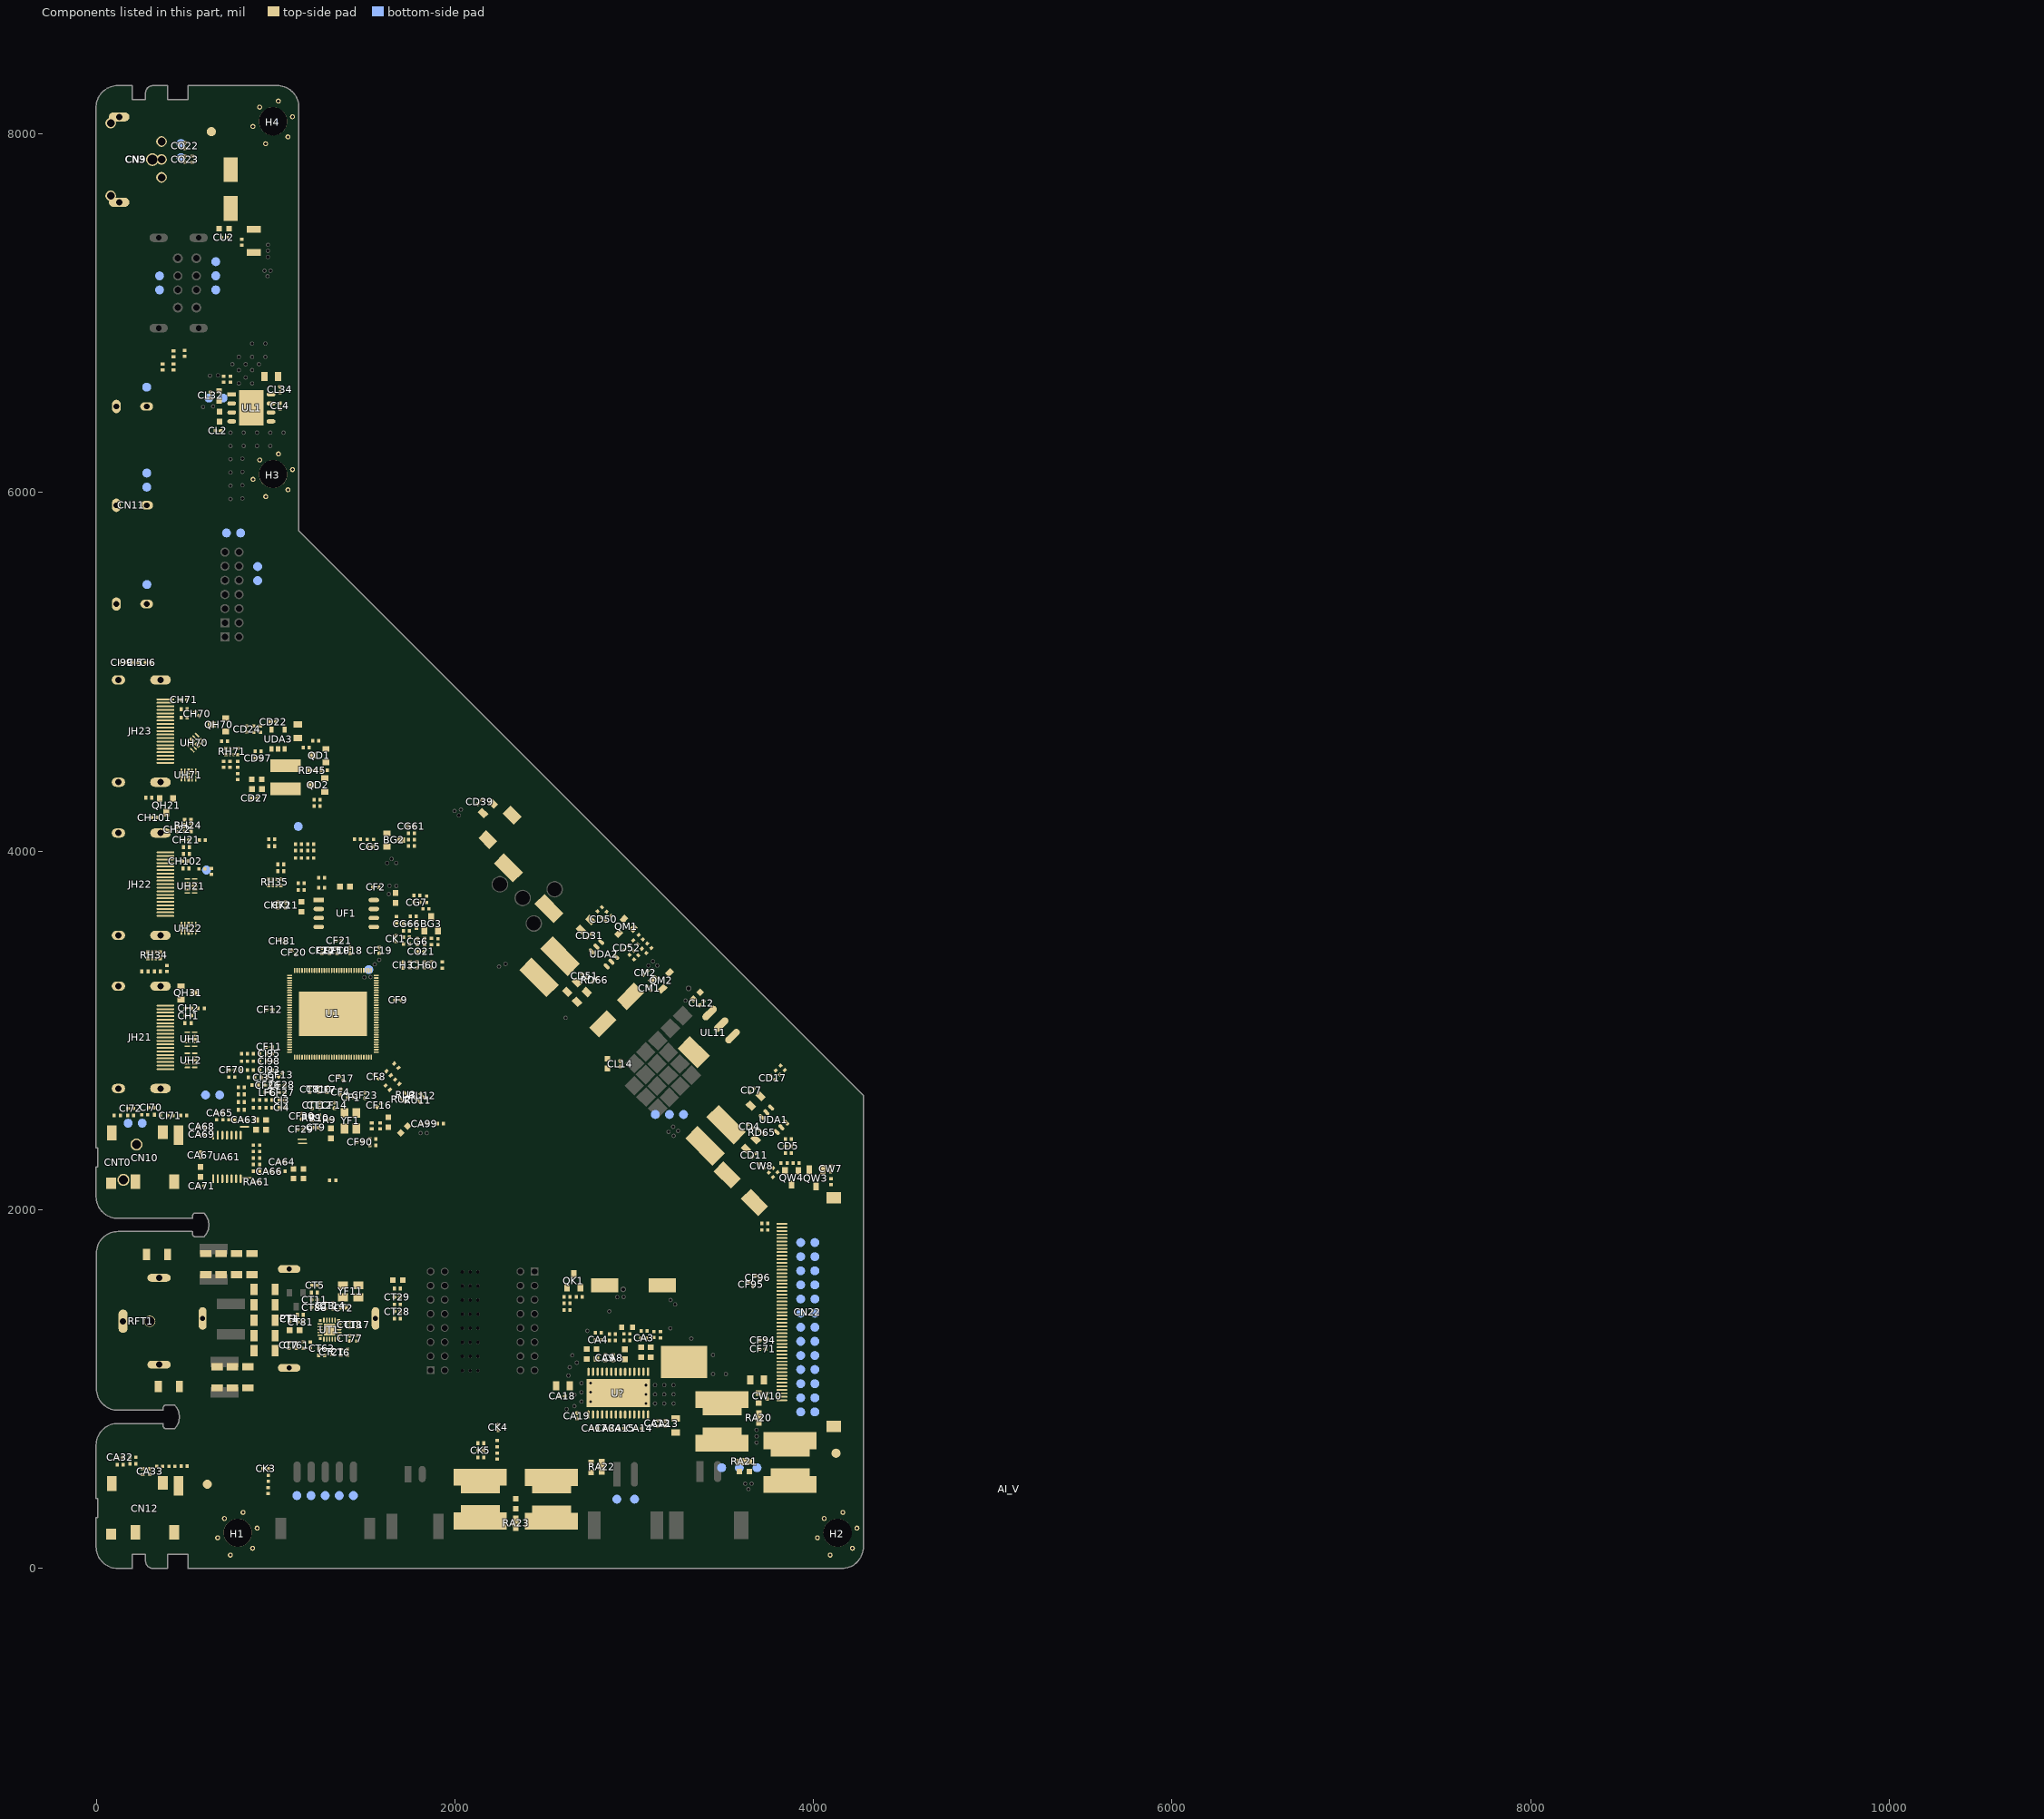
[diagram p0: the components of this part, seen from the top]
# Altium PCB MISC105950.PcbDoc (part 3 of 15)
Units mil, origin at the board's own origin, x right, y up, seen from the top; angles counter-clockwise.
Board outline 4280.62 x 8272.76 mil, 2 copper layers (TopLayer, BottomLayer), stack 61.855 mil thick; 541 components, 268 nets, 2324 pads, 1157 vias.

## Components (designator, comment, footprint, x,y, rotation, side; value= is the part's Value field where it differs from the comment) (continued)
LT4 "Ferrite bead,BEAD,1000ohm,0402,300mA,SMD,TRAY,CBM100505U102T,FH" L0402 1192.5,1243.5 r90 top
LT80 "NC/Multilayer inductor, HF Inductor, 270nH, ±5%, 0603, SMD, HCI1608F-R27J-M, Tai-tech" L0603 1105.5,1327 r0 top
M1 "MARK" MARK 617.5,467 r0 top
M2 "MARK" MARK 4125.5,640.5 r0 top
M3 "MARK" MARK 640,8013.5 r0 top
Manufacture_Info "Manufacture_Info" Manufacture_Info 2007.5,2940 r270 top
O0N "TEST" TP 4007.24,1815.64 r180 bottom
O0P "TEST" TP 3928.5,1815.64 r180 bottom
O1N "TEST" TP 4007.24,1736.9 r180 bottom
O1P "TEST" TP 3928.5,1736.9 r90 bottom
O2N "TEST" TP 4007.24,1658.16 r180 bottom
O2P "TEST" TP 3928.5,1658.16 r180 bottom
O3N "TEST" TP 4007.24,1500.68 r90 bottom
O3P "TEST" TP 3928.5,1500.68 r180 bottom
O4N "TEST" TP 4007.24,1421.94 r180 bottom
O4P "TEST" TP 3928.5,1421.94 r90 bottom
OCKN "TEST" TP 4007.24,1579.42 r90 bottom
OCKP "TEST" TP 3928.5,1579.42 r180 bottom
PT1 "NC/Shield cover, with seal, tinplate, T=0.3mm, natural color, 24.5×14×6mm, JLT" SHIELD(24.5*14*6)-TEMP-NG 1074,1392 r90 top locked
PWON "TEST" TP 898.43,5587.38 r90 bottom
QD1 "General-purpose transistor, Dynatron, PNP, 0.2A, 40V, 30-300, SOT-23, LMBT3906LT1G, LRC" SOT-23 1239.8,4532 r270 top
QD2 "General-purpose transistor, Dynatron, NPN, 0.2A, 40V, 30-300, SOT-23, LMBT3904LT1G, LRC" SOT-23 1233,4368.5 r270 top
QH21 "General-purpose transistor, Dynatron, NPN, 0.2A, 40V, 30-300, SOT-23, LMBT3904LT1G, LRC" SOT-23 389,4252.5 r0 top
QH31 "General-purpose transistor, Dynatron, NPN, 0.2A, 40V, 30-300, SOT-23, LMBT3904LT1G, LRC" SOT-23 511,3208.5 r90 top
QH70 "General-purpose transistor, Dynatron, NPN, 0.2A, 40V, 30-300, SOT-23, LMBT3904LT1G, LRC" SOT-23 680,4704.5 r270 top
QK1 "NC/MMBT3904(f≥350MHz)" SOT-23 2661.5,1602.5 r180 top
QM1 "General-purpose transistor, Dynatron, NPN, 0.2A, 40V, 30-300, SOT-23, LMBT3904LT1G, LRC" SOT-23 2940.5,3566 r315 top
QM2 "MOSFET, PMOS, -4.2A, -30V, 0.052ohm@ID=-4.2A@VGS=-10V, SOT-23-3, AO3401, BLUE ROCKET" SOT-23-1 3164,3290.5 r135 top
QW3 "MOSFET, PMOS, -4.3A, -30V, 0.048ohm@ID=-3A@VGS=-4.5V, SOT-23-3L, NCE3407AY, NCEPOWER" SOT-23-1 4013.84,2174.5 r0 top
QW4 "General-purpose transistor, Dynatron, NPN, 0.2A, 40V, 30-300, SOT-23, LMBT3904LT1G, LRC" SOT-23 3878,2176 r0 top
R9 "NC/0ohm-0402-PCB" R0402SC#2 1300,2500.5 r180 top
R10 "NC/0ohm-0402-PCB" R0402SC#1 1244,2511.77 r270 top
R99 "NC/0ohm-0402-PCB" R0402SC#1 1201.5,2511.77 r270 top
RA1 "4K7ohm-0402-±1%-1/16W" R0402 3145.5,1301 r270 top
RA2 "4K7ohm-0402-±1%-1/16W" R0402 3109,1301.5 r90 top
RA3 "1Kohm-0402-±1%-1/16W" R0402 3054,1322 r0 top
RA4 "NC/?" GND#1 1149.4,2368.34 r180 top
RA5 "NC/?" GND#1 1147.4,2392.34 r180 top
RA6 "Thick-film resistor, RES, 1/16W, 150ohm, ±1%, 0402, SMD" R0402 420.5,567.5 r180 top
RA7 "Thick-film resistor, RES, 1/10W, 200ohm, ±5%, 0603, SMD" R0603 2959.5,1342.5 r180 top
RA8 "100Kohm-0402-±1%-1/16W" R0402 2959.5,1306.5 r0 top
RA9 "NC/47Kohm-0402-±5%-1/16W" R0402 2959.5,1270 r0 top
RA10 "NC/10Kohm-0402-±1%-1/16W" R0402 2876.94,1269 r180 top
RA11 "NC/Thick-film resistor, RES, 1/16W, 13Kohm, ±1%, 0402, SMD" R0402 2876.94,1305.5 r180 top
RA14 "1Kohm-0402-±1%-1/16W" R0402 2799.02,1312.23 r180 top
RA15 "Thick-film resistor, RES, 1/16W, 150ohm, ±1%, 0402, SMD" R0402 203.5,580.5 r180 top
RA20 "NC/0ohm-0603-PCB" R0603SC 3694.5,837.5 r270 top
RA21 "NC/0ohm-0603-PCB" R0603SC 3612.5,594 r180 top
RA22 "NC/0ohm-0603-PCB" R0603SC 2818,565 r90 top
RA23 "NC/0ohm-0603-PCB" R0603SC 2339,250.22 r270 top
RA51 "47Kohm-0402-±1%-1/16W" R0402 957.5,432.5 r90 top
RA52 "10Kohm-0402-±1%-1/16W" R0402 1919,2478.5 r180 top
RA55 "1Kohm-0402-±1%-1/16W" R0402 203.5,618 r180 top
RA56 "1Kohm-0402-±1%-1/16W" R0402 352.5,567 r180 top
RA61 "NC/NC/0ohm-0402-PCB" R0402SC#1 892.5,2155 r180 top
RA62 "NC/47Kohm-0402-±5%-1/16W" R0402 755,2501 r180 top
RA63 "NC/47Kohm-0402-±5%-1/16W" R0402 1035,2213.5 r180 top
RA64 "NC/" GND#2 825.16,2461.54 r0 top
RA65 "NC/" GND#1 841,2176 r0 top
RA66 "NC/100Kohm-0402-±5%-1/16W" R0402 687.5,2501 r180 top
RA67 "NC/100Kohm-0402-±5%-1/16W" R0402 892.5,2213.5 r180 top
RA68 "NC/1Kohm-0402-±5%-1/16W" R0402 892.5,2323.75 r180 top
RA69 "NC/4K7ohm-0402-±5%-1/16W" R0402 892.5,2359.25 r180 top
RA70 "NC/12Kohm-0402-±5%-1/16W" R0402 1317.5,2162.5 r0 top
RA71 "NC/5K1ohm-0402-±5%-1/16W" R0402 892.5,2251.5 r0 top
RA72 "NC/12Kohm-0402-±5%-1/16W" R0402 892.5,2287.5 r180 top
RD1 "NC/10Kohm-0402-±5%-1/16W" R0402 3800.48,2764.52 r315 top
RD2 "100Kohm-0402-±1%-1/16W" R0402 900.27,4556.5 r0 top
RD28 "NC/4K7ohm-0402-±1%-1/16W" R0402 3827.15,2790.35 r135 top
RD31 "NC/Thick-film resistor, RES, 1/16W, 200Kohm, ±1%, 0402, SMD" R0402 3858.83,2314.54 r180 top
RD35 "NC/Thick-film resistor, RES, 1/16W, 10.5Kohm, ±1%, 0402, SMD" R0402 3859.27,2393 r0 top
RD42 "510ohm-0402-±1%-1/16W" R0402 1222,4615 r180 top
RD43 "4K7ohm-0402-±1%-1/16W" R0402 1170.27,4576.5 r0 top
RD44 "10Kohm-0402-±1%-1/16W" R0402 1271.3,4450 r180 top
RD45 "NC/0ohm-0402-PCB" R0402SC#1 1203.57,4450 r0 top
RD46 "10Kohm-0402-±1%-1/16W" R0402 1230.5,4251 r180 top
RD47 "NC/10Kohm-0402-±5%-1/16W" R0402 1230.5,4287 r0 top
RD52 "100Kohm-0402-±1%-1/16W" R0402 2807,3675 r45 top
RD53 "NC/Thick-film resistor, RES, 1/16W, 10Kohm, ±1%, 0402, SMD" R0402 2857.5,3649.5 r315 top
RD54 "Thick-film resistor, RES, 1/16W, 20Kohm, ±1%, 0402, SMD" R0402 3010,3406 r45 top
RD65 "NC/0ohm-0402-PCB" R0402SC#1 3711.5,2430.5 r315 top
RD66 "NC/0ohm-0402-PCB" R0402SC#1 2778,3279.5 r45 top
RD81 "12Kohm-0402-±1%-1/16W" R0402 877,4680 r270 top
RD88 "13Kohm-0402-±1%-1/16W" R0402 913,4680 r90 top
RD91 "Thick-film resistor, RES, 1/16W, 150Kohm, ±1%, 0402, SMD" R0402 2984.72,3432.6 r45 top
RF3 "NC/4K7ohm-0402-±5%-1/16W" R0402 1255,3795.5 r180 top
RF4 "NC/100ohm-0402-±5%-1/16W" R0402 3728,1922.27 r180 top
RF5 "NC/1Kohm-0402-±5%-1/16W" R0402 3728,1886 r0 top
RF12 "68ohm-0402-±5%-1/16W" R0402 884.5,2695 r180 top
RF13 "4K7ohm-0402-±1%-1/16W" R0402 1728.5,3518.5 r0 top
RF19 "68ohm-0402-±5%-1/16W" R0402 755,2738.5 r0 top
RF29 "4K7ohm-0402-±1%-1/16W" R0402 1766.5,3636.5 r180 top
RF43 "4K7ohm-0402-±1%-1/16W" R0402 1542.23,2393.5 r0 top
RF44 "4K7ohm-0402-±1%-1/16W" R0402 1542.23,2357.5 r0 top
RFT1 "RF connector, RF JACK, H, IEC, T14.5, CH6.3, with pipe, 23.8×15.1×11.9mm, SMD, 120-XX1, GD" T-12.8×10×9.3-IEC14.5-6.3 0.05,1376.72 r270 top locked
RG1 "10Kohm-0402-±1%-1/16W" R0402 1527.5,4064.5 r180 top
RG2 "NC/10Kohm-0402-±5%-1/16W" R0402 1784.5,3585 r270 top
RG3 "1Kohm-0402-±1%-1/16W" R0402 1729,3555.5 r180 top
RG6 "100ohm-0402-±1%-1/16W" R0402 1756.5,4063.75 r180 top
RG7 "NC/100ohm-0402-±5%-1/16W" R0402 1841,3730.5 r270 top
RG8 "NC/?" R0402 1756.5,4099.5 r0 top
RG9 "NC/NC/?" R0402 1786.5,3752 r0 top
RG29 "4K7ohm-0402-±1%-1/16W" R0402 1454.5,4065.5 r180 top
RG66 "1Kohm-0402-±1%-1/16W" R0402 1756.5,4028 r0 top
RG67 "NC/1Kohm-0402-±5%-1/16W" R0402 1838,3677.5 r180 top
RH1 "22Kohm-0402-±1%-1/16W" R0402 1929,3364 r90 top
RH2 "33Kohm-0402-±1%-1/16W" R0402 1868.5,3364.5 r90 top
RH23 "1Kohm-0402-±1%-1/16W" R0402 590.5,4061.5 r180 top
RH24 "Resistor array, RES ARRAY, 1/16W, 4×10Kohm, ±5%, 0402, SMD" RA0402 509.22,4142.34 r180 top
RH33 "1Kohm-0402-±1%-1/16W" R0402 583.5,3123 r0 top
RH34 "Resistor array, RES ARRAY, 1/16W, 4×10Kohm, ±5%, 0402, SMD" RA0402 320.54,3418.78 r270 top
RH35 "Resistor array, RES ARRAY, 1/16W, 4×33ohm, ±5%, 0402, SMD" RA0402 994,3826.5 r270 top
RH70 "1Kohm-0402-±1%-1/16W" R0402 714.5,4612 r180 top
RH71 "Resistor array, RES ARRAY, 1/16W, 4×10Kohm, ±5%, 0402, SMD" RA0402 754.34,4555.78 r90 top
RH72 "33ohm-0402-±1%-1/16W" R0402 708.5,4483 r270 top
RH73 "33ohm-0402-±1%-1/16W" R0402 744.5,4483 r270 top
RH74 "22Kohm-0402-±1%-1/16W" R0402 787.75,4483.26 r90 top
RH75 "33Kohm-0402-±1%-1/16W" R0402 787.75,4415.76 r270 top
RH81 "22Kohm-0402-±1%-1/16W" R0402 1786,3365.5 r90 top
RH82 "33Kohm-0402-±1%-1/16W" R0402 1749.5,3364.5 r90 top
RH83 "100ohm-0402-±1%-1/16W" R0402 587.5,3900 r180 top
RH101 "4K7ohm-0402-±1%-1/16W" R0402 1126.43,4002 r0 top
RH102 "Thick-film resistor, RES, 1/16W, 1.2Kohm, ±1%, 0402, SMD" R0402 1126.43,4037.75 r0 top
RH103 "1Kohm-0402-±1%-1/16W" R0402 1126.93,3961.25 r0 top
RH104 "4K7ohm-0402-±1%-1/16W" R0402 1194.43,3961.25 r0 top
RH105 "Thick-film resistor, RES, 1/16W, 220ohm, ±1%, 0402, SMD" R0402 1193.93,4037.75 r0 top
RH106 "NC/4K7ohm-0402-±5%-1/16W" R0402 1193.93,4002 r180 top
RI13 "10Kohm-0402-±1%-1/16W" R0402 892.5,2610 r180 top
RI14 "12Kohm-0402-±1%-1/16W" R0402 962.74,2610 r180 top
RI15 "10Kohm-0402-±1%-1/16W" R0402 892.5,2568 r180 top
RI16 "12Kohm-0402-±1%-1/16W" R0402 962.74,2568 r180 top
RI21 "75ohm-0402-±1%-1/16W" R0402 807,2682.5 r0 top
RI22 "33ohm-0402-±1%-1/16W" R0402 864.5,2736.5 r0 top
RI23 "75ohm-0402-±1%-1/16W" R0402 824.77,2869 r0 top
RI24 "33ohm-0402-±1%-1/16W" R0402 892,2869 r0 top
RI25 "75ohm-0402-±1%-1/16W" R0402 824.77,2778.5 r0 top
RI26 "33ohm-0402-±1%-1/16W" R0402 892,2778.5 r0 top
RI36 "75ohm-0402-±1%-1/16W" R0402 824.77,2827.5 r0 top
RI38 "33ohm-0402-±1%-1/16W" R0402 892,2827.5 r0 top
RI62 "Thick-film resistor, RES, 1/16W, 0ohm, ±1%, 0402, SMD" R0402 189,2524.5 r0 top
RI63 "Thick-film resistor, RES, 1/16W, 0ohm, ±1%, 0402, SMD" R0402 267.5,2528.5 r180 top
RK1 "22ohm-0402-±1%-1/16W" R0402 958,500 r90 top
RK2 "4K7ohm-0402-±1%-1/16W" R0402 2235.5,694 r270 top
RK6 "1Kohm-0402-±1%-1/16W" R0402 1673.5,3617 r270 top
RK10 "NC/1Kohm-0402-±5%-1/16W" R0402 2692.5,1512.5 r0 top
RK13 "NC/33Kohm-0402-±5%-1/16W" R0402 2624,1440 r0 top
RK14 "510ohm-0402-±1%-1/16W" R0402 2624.5,1512.5 r0 top
RK15 "NC/10Kohm-0402-±5%-1/16W" R0402 2624.5,1476.5 r0 top
RK23 "1Kohm-0402-±1%-1/16W" R0402 1255,3850 r0 top
RK25 "10Kohm-0402-±1%-1/16W" R0402 2235.5,624 r270 top
RL31 "120ohm-0402-±1%-1/16W" R0402 709.5,6632 r90 top
RL32 "200ohm-0402-±1%-1/16W" R0402 746.5,6632 r270 top
RM1 "10Kohm-0402-±1%-1/16W" R0402 3083.5,3471.5 r315 top
RM2 "10Kohm-0402-±1%-1/16W" R0402 3036.5,3519.5 r135 top
RM3 "4K7ohm-0402-±1%-1/16W" R0402 3006.5,3490.5 r315 top
RM4 "100Kohm-0402-±1%-1/16W" R0402 3054.5,3443 r315 top
RO21 "Thick-film resistor, RES, 1/16W, 150ohm, ±1%, 0402, SMD" R0402 1830,3495.5 r90 top
RO22 "NC/Thick-film resistor, RES, 1/16W, 75ohm, ±1%, 0402, SMD" R0402 1904.5,3495 r270 top
RO31 "Thick-film resistor, RES, 1/16W, 0ohm, ±1%, 0402, SMD" R0402 534,7859.38 r270 top
ROUT+ "DM0" TP 2902.57,384 r90 bottom
ROUT- "DM0" TP 3001,384 r90 bottom
RT1 "Thick-film resistor, RES, 1/16W, 51Kohm, ±1%, 0402, SMD" R0402 1255.5,1185.5 r180 top
RT2 "33ohm-0402-±1%-1/16W" R0402 1401,1204.5 r90 top
RT3 "33ohm-0402-±1%-1/16W" R0402 1452,1282 r90 top
RT4 "100ohm-0402-±1%-1/16W" R0402 1678.5,1391.5 r0 top
RT5 "100ohm-0402-±1%-1/16W" R0402 1677.5,1470.5 r0 top
RU1 "Thick-film resistor, RES, 1/16W, 0ohm, ±1%, 0402, SMD" R0402 809.38,7397.5 r270 top
RU2 "NC/0ohm-0402-PCB" R0402SC#1 1702.86,2614.64 r315 top
RU3 "NC/0ohm-0402-PCB" R0402SC#1 1728.38,2640.16 r315 top
RU11 "NC/0ohm-0402-PCB" R0402SC#1 1794.04,2608.96 r315 top
RU12 "NC/0ohm-0402-PCB" R0402SC#1 1819.33,2634.26 r315 top
RW10 "4K7ohm-0402-±1%-1/16W" R0402 3786.5,2219.5 r315 top
RW11 "NC/4K7ohm-0402-±5%-1/16W" R0402 4097.5,2156 r270 top
RW12 "47Kohm-0402-±1%-1/16W" R0402 3761.76,2193.47 r135 top
RW13 "4K7ohm-0402-±1%-1/16W" R0402 3835.27,2259.5 r0 top
RW14 "4K7ohm-0402-±1%-1/16W" R0402 3902.77,2259.5 r0 top
RXD "" TP 1125,4137.5 r270 bottom
S/N1 "Barcode" Barcode 2330.5,2498.5 r270 top
S/N2 "Barcode" Barcode 2465,2517 r90 bottom
SPDIF_OUT "TEST" TP 470.87,7947.38 r90 bottom
TXD "" TP 613,3894 r270 bottom
U1 "Customer-supplied TV main IC, IC Main Chip, SMD, TSUMV53RWU-Z1, COMPANY_A-ODM, MTK" QFN128/0.35-1 1318.5,3091.88 r0 top locked
U? "Audio amplifier, IC Audio, Class D, 2x10W@13V@8ohm, HTSSOP-28, SMD, CS3817EO, SEMICO" SSOP28/0.65-5 2910.2,975.41 r270 top
UA61 "NC/Audio amplifier, IC Headphone AMP, Class AB, 2×20mW@2.3V@32ohm, TSSOP-14, SMD, AD22653B-QH14NAR, ESMT" SSOP14/0.65-1 727.18,2293.06 r180 top locked
UDA1 "NC/DC-DC IC, IC DC-DC, Syn, 2A, 18V, 500kHz, SOT23-6, SMD, SM8102ABC, Silergy" SOT23-6-2 3778.5,2500.5 r45 top locked
UDA2 "DC-DC IC, IC DC-DC, Syn, 2A, 18V, 500kHz, SOT23-6, SMD, SM8102ABC, Silergy" SOT23-6-2 2830.5,3424.5 r45 top
UDA3 "DC-DC IC, IC DCDC, Syn, 1.2A, 6.0V, 1.5MHz, SOT23-5, SMD, TMI3408, TOLL" SOT-23-5 1012.5,4623.5 r0 top
UF1 "SPI flash IC, IC SPI FLASH, 4MB, 32Mb, SOIC8, SMD, W25Q32JVSSIQ, Winbond" SOIC8 1393.04,3651.5 r0 top locked
UH1 "NC/TVS diode, DIO ESD, 0.4pF, 19V, DFN2510-10L, SMD, ESD5304D-10/TR, Willsemi" RCL0524P 527,2950.38 r270 top
UH2 "NC/TVS diode, DIO ESD, 0.4pF, 19V, DFN2510-10L, SMD, ESD5304D-10/TR, Willsemi" RCL0524P 527,2832.38 r270 top
UH21 "NC/TVS diode, DIO ESD, 0.4pF, 19V, DFN2510-10L, SMD, ESD5304D-10/TR, Willsemi" RCL0524P 527,3804.71 r270 top
UH22 "NC/TVS diode, DIO ESD, 0.4pF, 19V, DFN2510-10L, SMD, ESD5304D-10/TR, Willsemi" RCL0524P 512.98,3569.5 r180 top
UH70 "NC/TVS diode, DIO ESD, 0.4pF, 19V, DFN2510-10L, SMD, ESD5304D-10/TR, Willsemi" RCL0524P 546.7,4605.01 r225 top
UH71 "NC/TVS diode, DIO ESD, 0.4pF, 19V, DFN2510-10L, SMD, ESD5304D-10/TR, Willsemi" RCL0524P 512.98,4423.83 r180 top
UL1 "LDO IC, IC LDO, 1A, 3.3V+ADJ, 12V, ESOP-8, SMD, LC1118CS8TRAD33, Leadchip" SOP8/1.27-3 863.5,6472 r0 top locked
UL11 "LDO IC, IC LDO, 1A, 1.8V, 15V, SOT-223, SMD, SCJT1117B-1.8V, CJKJ" SOT-223 3407.5,2955 r135 top
UT1 "Silicon tuner IC, IC Si Tuner, QFN-24, SMD, ATBM253, AltoBeam" QFN24/0.4-1 1299.5,1330 r90 top
VCC_CORE "TEST" TP 1518.5,3338.5 r315 bottom
VCC_PANEL1 "TEST" TP 3928.5,870.76 r90 bottom
XX.XXXX "PCB_NAME" PCB_NAME 1624.98,1044.62 r90 top
XXXXXX "PCB_TIME" PCB_TIME 8963.88,-1096.65 r90 top
XXXXXX. "PCB_TIME" PCB_TIME 1613.17,1044.62 r90 top
XXXXXXXX "PCB_NAME" PCB_NAME 8987.5,-1096.65 r90 top
XXXXXXXXXX "PCB_NAME" PCB_NAME 8952.07,-1096.65 r90 top
YF1 "Passive crystal oscillator, SPXO, 24MHz, ±10ppm, 12pF, SMD3225, SMD, SX32Y024000BC1T-Z, TKD" XTAL-S-3 1416.04,2495.51 r90 top
YF11 "Passive crystal oscillator, SPXO, 24MHz, ±10ppm, 12pF, SMD3225, SMD, SX32Y024000BC1T-Z, TKD" XTAL-S-3 1417,1543.5 r180 top locked
YPbPr_GND "TEST" TP 686.74,2639 r180 bottom
YPbPr_Pb "TEST" TP 254.5,2481.5 r180 bottom
YPbPr_Pr "TEST" TP 608,2639 r180 bottom
YPbPr_Y "TEST" TP 175.76,2481.5 r180 bottom
用U1上 "Glue, 0.1g, silicone, ZJ" "Heat-Shrinkable Tube" 8975.69,-1096.65 r90 top

## Footprints (in the part's own frame and the unit in brackets; to place one, negate y for a bottom-side part, rotate by r counter-clockwise, add the part's x,y. Pads: shape width x height; smd on the part's side, far side on the other; paste and mask are expansions set on the pad)
AI_GRIPPER_V [mm] "3D shape for vertical type AI equipment"
  round 1.5 on Mech5: 0(0,-2.5) 1(0,0) 2(0,2.5)
  body extent -29.13,-4.7 2.5,4.7, height 54.74
ASSE4.0C-3 [mm] "定位孔(顶底层上锡)(17.12.09更新过孔位置）18.11.22 更新paste形状为扇形。"
  round 4 hole 4 unplated mask+0: 0(0,0)
  round 0.7 hole 0.4: 1(-2.85,-0.725) 2(-1.893,2.011) 3(0.75,2.875) 4(2.75,0.65) 5(2.105,-2.203) 6(-1.05,-3.175)
  KeepOutLayer pour cut-out: 0,-2.3 -0.88,-2.125 -1.626,-1.626 -2.125,-0.88 -2.3,0 -2.3,0 -2.125,0.88 -1.626,1.626 -0.88,2.125 0,2.3 0,2.3 0.88,2.125 1.626,1.626 2.125,0.88 2.3,0 2.3,0 2.125,-0.88 1.626,-1.626 0.88,-2.125 0,-2.3
AV1-H-4-S [mm] "CS,RCA-143P-EP-07（通孔回流）,中心高度5.5.17.11.22"
  rect 3.6x4.3 on Top Paste: 0(-5.95,3.2) 0(5.95,3.2)
  rect 2.4x4.5 on Top Paste: 0(0,7.3)
  round 1.8 hole 1.4 mask+0.076: 1(0,7.9)
  oval 1.3x2.9 hole 0.9 slot 2.5 at 90 deg mask+0.076: 2(6.05,3.2) 3(-6.05,3.2)
  silkscreen extent -6.4,0 6.4,8.51, body extent -6.25,-9.1 6.25,8.4, height 10.25
AV3-H14-15-S [mm] "宇球；RC075-F03L3BY-D(SMD)中心高度：5.5mm;160427（17.09.20更新钢网）"
  rect 3.2x2.7 on Top Paste: 0(-14,2.8) 0(0,2.8) 0(14,2.8)
  rect 2.7x3.2 on Top Paste: 0(-14,7.1) 0(0,7.1) 0(14,7.1)
  oval 1.2x1.8 hole 0.8 slot 1.4 at 90 deg mask+0.076: 1(-14,7.1) 3(0,7.1) 5(14,7.1)
  oval 1.9x1.2 hole 0.8 slot 1.5 at 0 deg mask+0.076: 2(-14,2.8) 4(0,2.8) 6(14,2.8)
  silkscreen extent -20.3,0 20.3,7.8, body extent -21.25,-56.32 21.25,7.6, height 12.95
Barcode [mm]
  round 0.3 on Mech2: 0(0,0)
  silkscreen extent -15,-4 15,4
C0402 [mm] "片式电容  2018.10.7 替换为兼容0201封装"
  rrect50% 0.45x0.5 smd mask+0.051: 1(-0.425,0) 2(0.425,0)
  rect 0.3x0.3 smd mask+0.051: 1(-0.25,0) 2(0.25,0)
  rect 0.6x0.6 on Top Solder: 2(0,0)
  TopLayer pour cut-out: -0.318,0.302 -0.318,-0.303 0.306,-0.303 0.306,0.302
  silkscreen extent -0.87,-0.47 0.87,0.47, body extent -0.5,-0.25 0.5,0.25, height 0.5
C0603 [mm] "片式电容"
  rect 0.8x0.8 smd mask+0.076: 1(-0.706,0) 2(0.706,0)
  silkscreen extent -1.39,-0.62 1.39,0.62, body extent -0.8,-0.4 0.8,0.4, height 0.8
C0805 [mm] "片式电容"
  rect 0.9x1.25 smd mask+0.076: 1(-0.966,0) 2(0.966,0)
  silkscreen extent -1.73,-0.84 1.73,0.84, body extent -1,-0.62 1,0.63, height 1.25
C1206 [mm] "片式电容"
  rect 1x1.6 smd mask+0.076: 1(-1.5,0) 2(1.5,0)
  silkscreen extent -2.39,-1.02 2.39,1.02, body extent -1.6,-0.8 1.6,0.8, height 1.3
CQC [mil]
DIODE-S0402 [mm] "DVD上使用的ESD"
  rect 0.45x0.55 smd mask+0.051: A(-0.425,0) K(0.425,0)
  silkscreen extent -0.8,-0.43 0.91,0.43, body extent -0.5,-0.25 0.5,0.25, height 0.5
DIODE-SMB-2 [mm] "乐山无线电,SMBFJ12A，20161124"
  rect 1.6x2.2 smd: A(2.45,0) K(-2.45,0)
  silkscreen extent -2.35,-1.9 2.35,2.77, body extent -2.79,-1.91 2.79,1.91, height 1.4
DOLBY_AS2 [mil] "杜比认证预留框，两行印刷，规格35.0*5.4mm"
EC(6.5*5.5)-S [mm] "珠海华冠电容 100uF/16V  200UF/16V高度7.0mm"
  rect 2x3.5 smd: 1(0,2.75) 2(0,-2.75)
  silkscreen extent -3.4,-3.4 3.4,3.4, body extent -4.55,-4.59 4.62,4.58, height 5.41
EC(10*10.5)-S [mm] "RV330M100G105ETR ;15.07.27"
  rect 2x3.85 smd: 1(0,4.075) 2(0,-4.075)
  silkscreen extent -5.25,-5.23 5.25,5.28, body extent -5.25,-5.25 5.28,5.28, height 11.1
FFC51H/0.5S-8 [mm] "昶通;FPC 0.5Pitch 51P（30P-96P）前掀式(翻开高度6.8mm);160710"
  oval 0.25x1.55 smd: 1(-12.5,3.675) 2(-12,3.675) 3(-11.5,3.675) 4(-11,3.675) 5(-10.5,3.675) 6(-10,3.675) 7(-9.5,3.675) 8(-9,3.675) 9(-8.5,3.675) 10(-8,3.675) 11(-7.5,3.675) 12(-7,3.675) 13(-6.5,3.675) 14(-6,3.675) 15(-5.5,3.675) 16(-5,3.675) 17(-4.5,3.675) 18(-4,3.675) 19(-3.5,3.675) 20(-3,3.675) 21(-2.5,3.675) 22(-2,3.675) 23(-1.5,3.675) 24(-1,3.675) 25(-0.5,3.675) 26(0,3.675) 27(0.5,3.675) 28(1,3.675) 29(1.5,3.675) 30(2,3.675) 31(2.5,3.675) 32(3,3.675) 33(3.5,3.675) 34(4,3.675) 35(4.5,3.675) 36(5,3.675) 37(5.5,3.675) 38(6,3.675) 39(6.5,3.675) 40(7,3.675) 41(7.5,3.675) 42(8,3.675) 43(8.5,3.675) 44(9,3.675) 45(9.5,3.675) 46(10,3.675) 47(10.5,3.675) 48(11,3.675) 49(11.5,3.675) 50(12,3.675) 51(12.5,3.675)
  rect 1.6x2.1 smd: 52(16.2,-3.675) 53(-16.2,-3.675)
  silkscreen extent -16.35,-5.81 16.35,5.4
FIX-5.5*7.0*7.8-S-1 [mm] "薪祥,Φ5.5×7.0×7.8mm-M3,中心高度:4mm,0726_2018,图纸变更:将2PIN向下挪1.85mm,0728_2018"
  rect 3.3x3 on Top Paste: 0(-2.25,5.65)
  oval 1.4x0.9 on Keep-Out: 0(0,0.35)
  rect 3.3x1.4 on Top Paste: 0(2.25,3.4)
  round 1.7 hole 1.3 mask+0.076: 1(-2.5,5.65) 2(2.5,3.8)
  silkscreen extent -2.85,0 2.85,8
FUSE1.1A-S [mm] "保险丝：FSMD005-1206(FUZETEC)（兼容1206F8.00A063V 高度0.8mm），18.03.07）"
  rect 1x2 smd: 1(-1.65,0) 2(1.65,0)
  silkscreen extent -2.4,-1.2 2.4,1.2, body extent -1.75,-0.9 1.75,0.9, height 1
GND#1 [mm] "导通线"
  rect 0.66x0.178 smd paste-0.45 mask-0.45: JP_1K(-0.32,0) JP_2K(0.32,0)
GND#2 [mm] "导通线"
  rect 0.66x0.3 smd paste-0.45 mask-0.45: JP_1K(-0.32,0) JP_2K(0.32,0)
HDMI-HS-1 [mm] "浙江和丰   HHF-14B000-2SA。17.09.25更新钢网;171107更新焊盘露铜位置;18.04.19 更新大脚孔径;19.09.11 更新端子视图开口高度(6.1-6.2,0."
  rect 2.2x3.8 on Top Paste: 0(-7.75,4.18) 0(7.753,4.183)
  rect 2.2x6 on Top Paste: 0(-7.75,9.355) 0(7.75,9.355)
  oval 0.26x2.5 smd: 1(4.5,11.258) 2(4,11.258) 3(3.5,11.258) 4(3,11.258) 5(2.5,11.258) 6(2,11.258) 7(1.5,11.258) 8(1,11.258) 9(0.5,11.258) 10(0,11.258) 11(-0.5,11.258) 12(-1,11.258) 13(-1.5,11.258) 14(-2,11.258) 15(-2.5,11.258) 16(-3,11.258) 17(-3.5,11.258) 18(-4,11.258) 19(-4.5,11.258)
  oval 1.3x2.9 hole 0.9 slot 2.5 at 90 deg mask+0.076: 20(-7.25,10.565) 22(7.25,10.55)
  oval 1.3x1.9 hole 0.9 slot 1.5 at 90 deg mask+0.076: 21(-7.25,4.59) 23(7.25,4.59)
  silkscreen extent -7.5,2 7.5,12.19, body extent -10.25,-57.68 10.25,12.17, height 8.92
"Heat-Shrinkable Tube" [mm] "收缩前壁厚0.3+-0.05，收缩后壁厚0.6+-0.1"
  round 0.3 on Mech2: 0(0,0)
HL030 [mm] "P.CPP.200BP.2 A14491汇流条-(6*4mm)-不常用"
  rect 6.6x4.6 smd: 1(0,0)
  silkscreen extent -3.8,-2.8 3.8,2.8, body extent -3,-2 3,2, height 1
HS(15X15X5)-S [mil] "YT.YT-P-151505.2019/9/18"
  silkscreen extent -300,-300 300,300, body extent -295,-295 295,295, height 197
L0402 [mm] "电感"
  rect 0.45x0.55 smd mask+0.076: 1(-0.425,0) 2(0.425,0)
  silkscreen extent -0.8,-0.42 0.8,0.43, body extent -0.5,-0.25 0.5,0.25, height 0.5
L0603 [mil] "片式磁珠、电感、ESD"
  rect 32x31.5 smd mask+3: 1(-27.81,0) 2(27.81,0)
  silkscreen extent -50,-22 50,22, body extent -31,-16 31,16, height 31
L(4.5*3.5)-S [mm] "SMD4532-6R8M-023"
  rect 1.8x4.3 smd: 1(-1.65,0) 2(1.65,0)
  TopLayer pour cut-out: -0.76,2.15 0.796,2.15 0.796,2.141 0.796,-2.149 -0.756,-2.149 -0.756,-2.15
  silkscreen extent -2.83,-2.44 3.3,2.44
L(5.8*4.5)-S [mm] "APC52A45M4R7\电感\Cailank;170317更新阻焊兼容L(4*3.0)-S"
  rect 2.5x5.5 smd paste-5.5: 1(2.105,0) 2(-2.105,0)
  TopLayer pour cut-out: -0.849,2.746 -0.845,2.75 0.861,2.75 0.861,-2.749 0.861,-2.753 0.859,-2.753 -0.862,-2.753
  silkscreen extent -1.5,-2.9 3.88,2.9, body extent -3.06,-2.65 3.08,2.74, height 4.8
L(5.8*4.5)-S-3 [mm] "APC52A45M4R7\电感\Cailank,与0805磁珠兼容,有方向"
  rect 2.5x5.5 smd paste-5 mask-5: F(2.105,0) S(-2.105,0)
  TopLayer pour cut-out: -0.849,2.746 -0.845,2.75 0.861,2.75 0.861,-2.749 0.861,-2.753 0.859,-2.753 -0.862,-2.753
  silkscreen extent -1.5,-2.9 1.5,2.9, body extent -3.06,-2.65 3.08,2.74, height 4.8
L(8*4.2)-S [mm] "SWPA8040S,电感"
  rect 2.4x7.5 smd paste-7 mask-7: 1(3.1,0) 2(-3.1,0)
  TopLayer pour cut-out: -1.906,3.75 -1.906,3.75 1.907,3.75 1.907,-3.749 1.907,-3.75 -1.91,-3.75
  silkscreen extent -4.5,-4.15 5,4.15, body extent -4,-4 4,4, height 4.2
Manufacture_Info [mm]
  round 0.3 on Mech2: 0(0,0)
MARK [mm] "SMD 使用"
  round 1.3 smd paste+0 mask+0.65: 0(0,0)
  TopLayer circle w0.254: c0,0 r1.444
  TopLayer pour cut-out: -1.3,0 -1.201,-0.497 -0.919,-0.919 -0.497,-1.201 0,-1.3 0,-1.3 0.497,-1.201 0.919,-0.919 1.201,-0.497 1.3,0 1.3,0 1.201,0.497 0.919,0.919 0.497,1.201 0,1.3 0,1.3 -0.497,1.201 -0.919,0.919 -1.201,0.497 -1.3,0
"NO DOLBY-SILK" [mil]
  silkscreen extent -16,-177 1441,197
OPTICAL-HS-1 [mm] "广业,182500122,通孔回流，16.09.23(17.09.15更新钢网）(18.04.16 更新前视图）"
  rect 2.7x3 on Top Paste: 0(-4.875,2.7) 0(4.875,2.7)
  rect 2.5x4.1 on Top Paste: 0(-2.75,9.2) 0(0,9.2) 0(2.75,9.2)
  round 1.5 hole 1.1 mask+0.076: 1(-2.54,9.2) 2(0,9.2) 3(2.54,9.2) 4(5.15,2) 5(-5.15,2)
  silkscreen extent -6.28,0 6.28,11.41, body extent -6.15,-1.8 6.15,11.3, height 11.2
PCB_NAME [mm]
  round 0.3 on Mech2: 0(0,0)
PCB_TIME [mm]
  round 0.3 on Mech2: 0(0,0)
PHONE-HS-29 [mm] "JSL,PJ-342F,0702_2018"
  round 1.5 on Keep-Out: 0(0,9.5) 0(0,2.5)
  rect 1.6x1.4 smd mask+0.051: 1(3.7,2.05)
  rect 2.1x1.4 smd mask+0.051: 2(-3.45,2.15) 3(3.45,5.5) 5(3.45,11)
  rect 1.9x1.4 smd mask+0.051: 4(-3.55,9.4)
  rect 2.75x1.4 smd mask+0.051: 6(-3.125,11.6)
  TopLayer pour cut-out: 0.6,3.8 3.2,3.8 3.2,4.75 2.35,4.75 2.35,6.25 3.2,6.25 3.2,10.25 2.35,10.25 2.35,11.7 1.7,11.7 1.7,8.625 0.6,7.525
  TopLayer pour cut-out: -3.2,13.125 -1.475,13.125 -1.475,12.35 -3.2,12.35 -3.2,12.68
  TopLayer pour cut-out: -2.325,10.85 -2.325,10.15 -3.2,10.15 -3.2,10.85
  TopLayer pour cut-out: -3.2,3.975 -0.775,3.975 -0.775,0.825 -3.2,0.825 -3.2,1.375 -3.2,1.4 -2.35,1.4 -2.35,2.9 -3.2,2.9
  KeepOutLayer lines w0.051: 1.4,0.2 -1.4,0.2
  silkscreen extent -3.3,0 3.3,13.13, body extent -4,-2 4,13, height 4.75
QFN24/0.4-1 [mm] "Si2151;14-03-17;161116新增两个EPAD孔"
  rect 0.4x0.4 smd: 1(-1.295,1.295) 7(-1.295,-1.295) 13(1.295,-1.295) 19(1.295,1.295)
  oval 0.7x0.2 smd: 2(-1.35,0.8) 3(-1.35,0.4) 4(-1.35,0) 6(-1.35,-0.8) 14(1.35,-0.8) 15(1.35,-0.4) 16(1.35,0) 17(1.35,0.4) 18(1.35,0.8)
  oval 0.7x0.2 smd paste+0: 5(-1.35,-0.4)
  oval 0.2x0.7 smd: 8(-0.8,-1.35) 9(-0.4,-1.35) 10(0,-1.35) 11(0.4,-1.35) 12(0.8,-1.35) 20(0.8,1.35) 21(0.4,1.35) 22(0,1.35) 23(-0.4,1.35)
  oval 0.2x0.7 smd paste+0: 24(-0.8,1.35)
  rect 1.651x1.651 smd paste-2 mask-2: EPAD(0,0)
  silkscreen extent -2.6,-2.24 2.11,2.24, body extent -1.5,-1.5 1.5,1.5, height 0.9